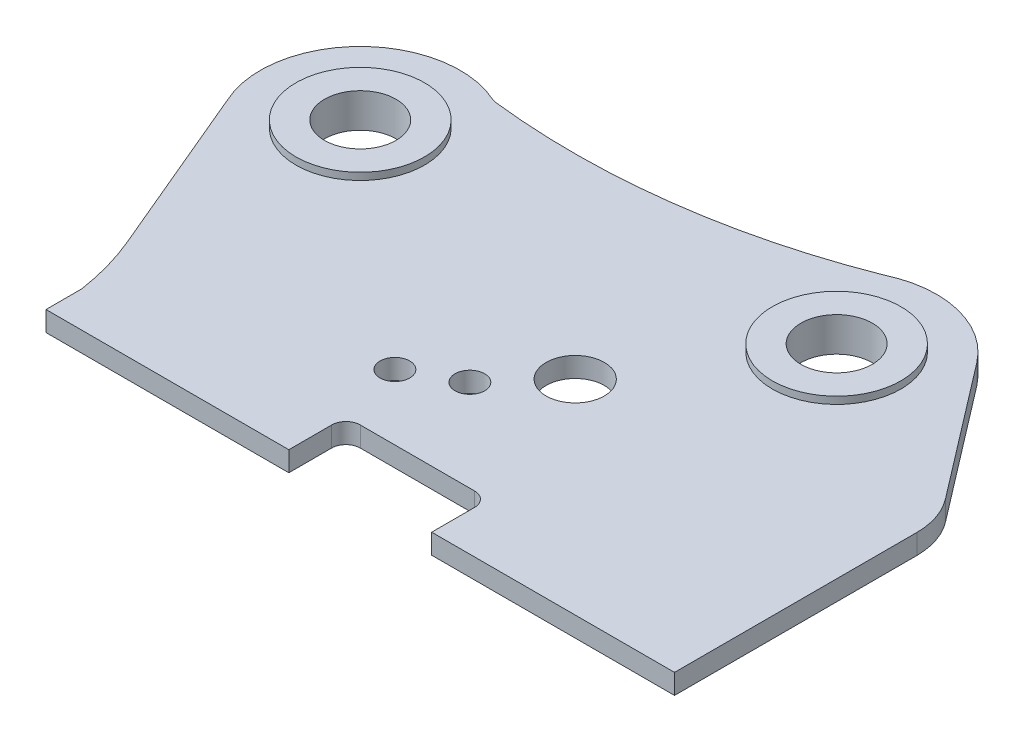
from build123d import *

# Parameters (mm, degrees)
SKETCH1_R             = 20.75
SKETCH1_R_2           = 90
SKETCH1_R_3           = 40.75
BOSS_EXTRUDE1_DEPTH   = 28
SKETCH_2_2_R          = 90
SKETCH_2_2_R_2        = 50
BOSS_EXTRUDE2_DEPTH   = 10
BOSS_EXTRUDE2_2_DEPTH = 10
BOSS_EXTRUDE3_START   = -38
SKETCH_2_2_2_R        = 90
SKETCH_2_2_2_R_2      = 50
BOSS_EXTRUDE3_DEPTH   = 38


with BuildPart() as part:
    # Sketch1 → Boss-Extrude1 (new body)
    with BuildSketch(Plane(origin=(0, 0, 0), x_dir=(1, 0, 0), z_dir=(0, 1, 0))):
        with BuildLine():
            Line((1925.70113656, 1748.394060435), (2027.880227878, 1505.832022369))
            ThreePointArc((2027.880227878, 1505.832022369), (2043.18353175, 1462.087406566), (2052.944070187, 1416.782722365))
            Line((2052.944070187, 1416.782722365), (2052.944070187, 1366.782722365))
            Line((2052.944070187, 1366.782722365), (2392.944070187, 1366.782722365))
            Line((2392.944070187, 1366.782722365), (2392.944070187, 1426.782722365))
            ThreePointArc((2392.944070187, 1426.782722365), (2398.801934564, 1440.924857989), (2412.944070187, 1446.782722365))
            Line((2412.944070187, 1446.782722365), (2572.944070187, 1446.782722365))
            ThreePointArc((2572.944070187, 1446.782722365), (2587.086205811, 1440.924857989), (2592.944070187, 1426.782722365))
            Line((2592.944070187, 1426.782722365), (2592.944070187, 1366.782722365))
            Line((2592.944070187, 1366.782722365), (2932.944070187, 1366.782722365))
            Line((2932.944070187, 1366.782722365), (2932.944070187, 1705.998908982))
            ThreePointArc((2932.944070187, 1705.998908982), (2927.653962259, 1738.093088264), (2912.343343312, 1766.791634101))
            Line((2912.343343312, 1766.791634101), (2769.10349201, 1953.872243723))
            ThreePointArc((2769.10349201, 1953.872243723), (2690.844558049, 2004.841768703), (2597.944509636, 1995.253534964))
            ThreePointArc((2597.944509636, 1995.253534964), (2361.126178322, 1934.317555647), (2116.599187921, 1932.684586999))
            ThreePointArc((2116.599187921, 1932.684586999), (2113.568985738, 1933.277336612), (2110.666130639, 1934.329434346))
            ThreePointArc((2110.666130639, 1934.329434346), (1953.690461842, 1905.518335141), (1925.70113656, 1748.394060435))
        make_face()
        with Locations(Location((2369.944070187, 1538.282722365, 0), (0, 0, 270))):
            Circle(SKETCH1_R, mode=Mode.SUBTRACT)
        with Locations(Location((2437.944070187, 1575.282722365, 0), (0, 0, 270))):
            Circle(SKETCH1_R, mode=Mode.SUBTRACT)
        with Locations(Location((2052.944070187, 1806.782722365, 0), (0, 0, 270))):
            Circle(SKETCH1_R_2, mode=Mode.SUBTRACT)
        with Locations(Location((2657.944509636, 1868.762428557, 0), (0, 0, 270))):
            Circle(SKETCH1_R_2, mode=Mode.SUBTRACT)
        with Locations(Location((2507.944070187, 1652.782722365, 0), (0, 0, 270))):
            Circle(SKETCH1_R_3, mode=Mode.SUBTRACT)
    extrude(amount=BOSS_EXTRUDE1_DEPTH)



with BuildPart() as body_2:
    # Sketch 2_2 → Boss-Extrude2 (new body)
    with BuildSketch(Plane(origin=(0, 28, 0), x_dir=(1, 0, 0), z_dir=(0, 1, 0))):
        with Locations(Location((2052.944070187, 1806.782722365, 0), (0, 0, 270))):
            Circle(SKETCH_2_2_R)
        with Locations(Location((2052.944070187, 1806.782722365, 0), (0, 0, 270))):
            Circle(SKETCH_2_2_R_2, mode=Mode.SUBTRACT)
    extrude(amount=BOSS_EXTRUDE2_DEPTH)


with BuildPart() as body_3:
    # Sketch 2_2 → Boss-Extrude2 2 (new body)
    with BuildSketch(Plane(origin=(0, 28, 0), x_dir=(1, 0, 0), z_dir=(0, 1, 0))):
        with Locations(Location((2657.944509636, 1868.762428557, 0), (0, 0, 270))):
            Circle(SKETCH_2_2_R)
        with Locations(Location((2657.944509636, 1868.762428557, 0), (0, 0, 270))):
            Circle(SKETCH_2_2_R_2, mode=Mode.SUBTRACT)
    extrude(amount=BOSS_EXTRUDE2_2_DEPTH)


with BuildPart() as part_1:
    add(part.part)

    add(body_2.part)  # Boss-Extrude3 merges body 2

    add(body_3.part)  # Boss-Extrude3 merges body 3
    # Sketch 2_2 2 → Boss-Extrude3 (add)
    # profile 1 of 2: a face of its own
    with BuildSketch(Plane(origin=(0, 28, 0), x_dir=(1, 0, 0), z_dir=(0, 1, 0)).offset(BOSS_EXTRUDE3_START)):
        with Locations(Location((2052.944070187, 1806.782722365, 0), (0, 0, 270))):
            Circle(SKETCH_2_2_2_R)
        with Locations(Location((2052.944070187, 1806.782722365, 0), (0, 0, 270))):
            Circle(SKETCH_2_2_2_R_2, mode=Mode.SUBTRACT)
    # profile 2 of 2: a face of its own
    with BuildSketch(Plane(origin=(0, 28, 0), x_dir=(1, 0, 0), z_dir=(0, 1, 0)).offset(BOSS_EXTRUDE3_START)):
        with Locations(Location((2657.944509636, 1868.762428557, 0), (0, 0, 270))):
            Circle(SKETCH_2_2_2_R)
        with Locations(Location((2657.944509636, 1868.762428557, 0), (0, 0, 270))):
            Circle(SKETCH_2_2_2_R_2, mode=Mode.SUBTRACT)
    extrude(amount=BOSS_EXTRUDE3_DEPTH)


solid = part_1.part
